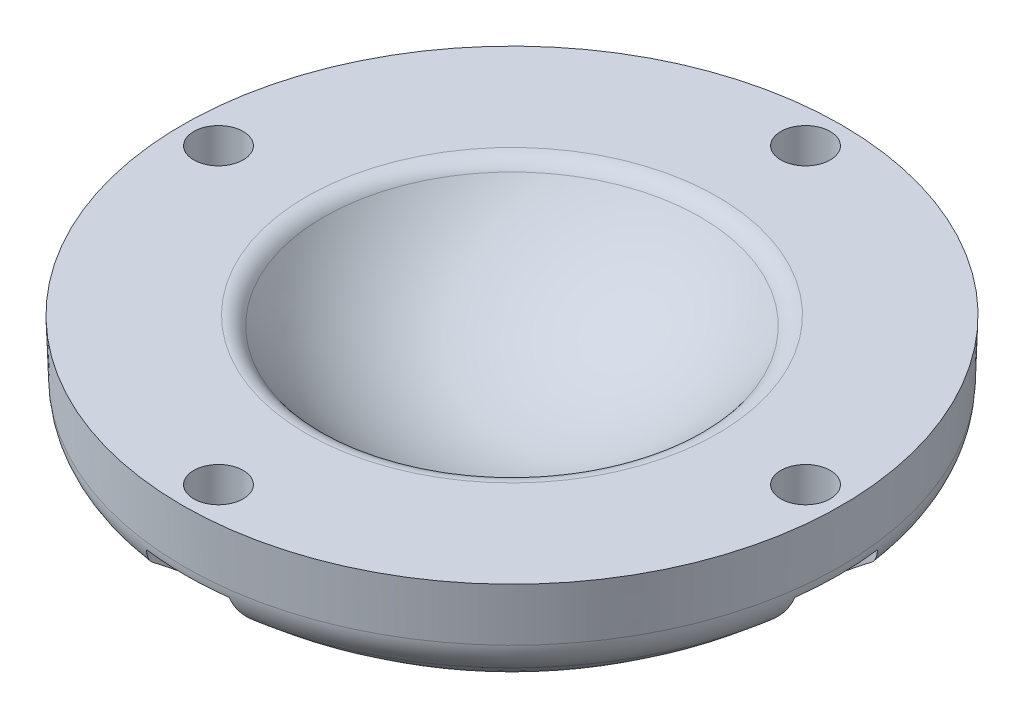
from build123d import *

# Parameters (mm, degrees)
HOLE_WIZARD_M2_1_D           = 2.4
HOLE_WIZARD_M2_1_CBORE_D     = 5
HOLE_WIZARD_M2_1_CBORE_DEPTH = 7


with BuildPart() as part:
    # 草图1 → 旋转1 (revolve)
    with BuildSketch(Plane.XY, mode=Mode.PRIVATE) as revolve_1_sk:
        with BuildLine():
            Line((0, -11), (0, -15.5))
            ThreePointArc((0, -15.5), (8.144809073, -14.009581241), (15.234037604, -9.731485667))
            ThreePointArc((15.234037604, -9.731485667), (15.718094855, -9.086559789), (15.908120336, -8.302894602))
            Line((15.908120336, -8.302894602), (16, -5.671805268))
            Line((16, -5.671805268), (9.974317744, -5.671805268))
            ThreePointArc((9.974317744, -5.671805268), (9.503140374, -5.789766785), (9.143124599, -6.115821496))
            ThreePointArc((9.143124599, -6.115821496), (5.182951068, -9.702423317), (0, -11))
        make_face()
    revolve(revolve_1_sk.sketch.rotate(Axis((0, -11, 0), (0, -1, 0)), 90), axis=Axis((0, -11, 0), (0, -1, 0)))

    # M2 六角头螺栓的柱形沉头孔1 (through all)
    with Locations(Plane.XZ.offset(15.671805268)):
        with Locations((-14.25, 0), (0, -14.25), (14.25, 0), (0, 14.25)):
            CounterBoreHole(HOLE_WIZARD_M2_1_D / 2, HOLE_WIZARD_M2_1_CBORE_D / 2, HOLE_WIZARD_M2_1_CBORE_DEPTH)


solid = part.part
